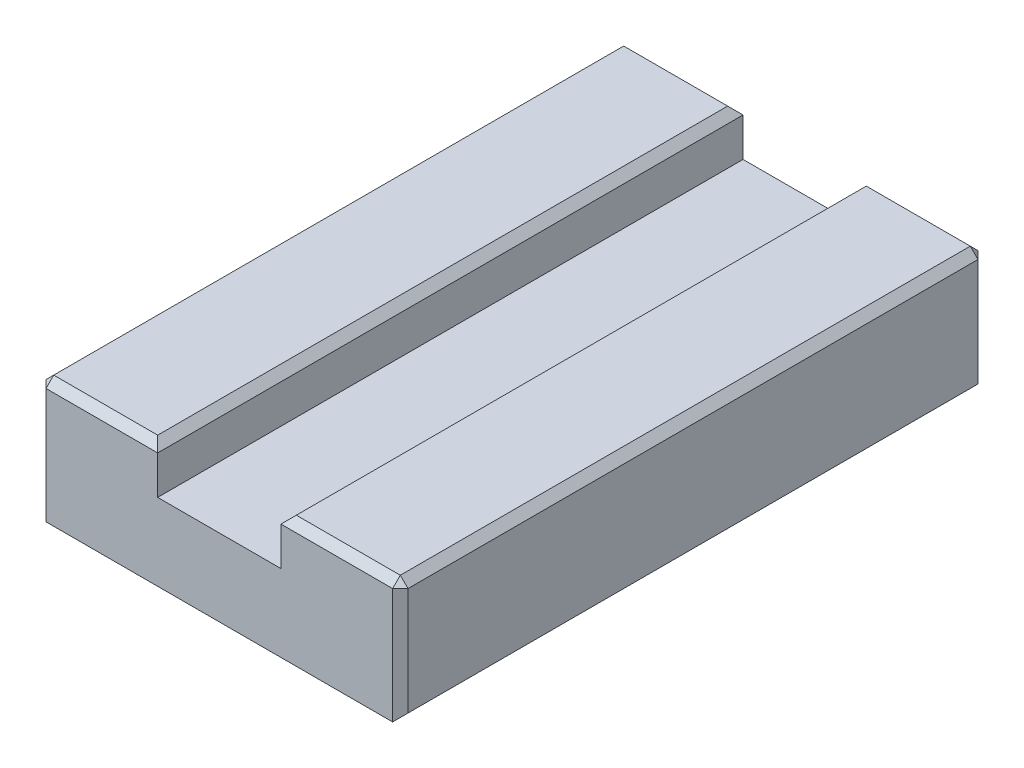
SolidWorks part; units mm, degrees
ref_plane "Front Plane" through (0, 0, 0) normal (0, 0, 1) x (1, 0, 0)
ref_plane "Top Plane" through (0, 0, 0) normal (0, 1, 0) x (1, 0, 0)
ref_plane "Right Plane" through (0, 0, 0) normal (1, 0, 0) x (0, 0, -1)
sketch "Sketch1" plane through (0, 0, 0) normal (0, 0, 1) x (1, 0, 0)
  line L0 (0, 22.704) -> (0, -28.0863) construction
  line L1 (-11.75, 4) -> (-4, 4)
  line L2 (-11.75, 4) -> (-11.75, -4)
  line L3 (-11.75, -4) -> (11.75, -4)
  line L4 (11.75, 4) -> (11.75, -4)
  line L5 (-11.75, 4) -> (11.75, -4) construction
  line L6 (-11.75, -4) -> (11.75, 4) construction
  line L7 (-4, 4) -> (-4, 1)
  line L8 (-4, 1) -> (4, 1)
  line L9 (4, 1) -> (4, 4)
  line L10 (4, 4) -> (11.75, 4)
  point P0 (0, 0)
  dimension "D1" = 23.5
  dimension "D2" = 8
  dimension "D3" = 8
  dimension "D4" = 3
extrude "Boss-Extrude1" add sketch "Sketch1" along normal blind 38
chamfer "Chamfer1" distance 0.5 angle 45 14 edges at (11.75, -4, 19) (11.75, 0, 38) (11.75, 0, 0) (11.75, 4, 19) (7.875, 4, 38) (4, 4, 19) (7.875, 4, 0) (-11.75, 0, 38) (-11.75, -4, 19) (-11.75, 0, 0) (-4, 4, 19) (-7.875, 4, 38) (-11.75, 4, 19) (-7.875, 4, 0)
